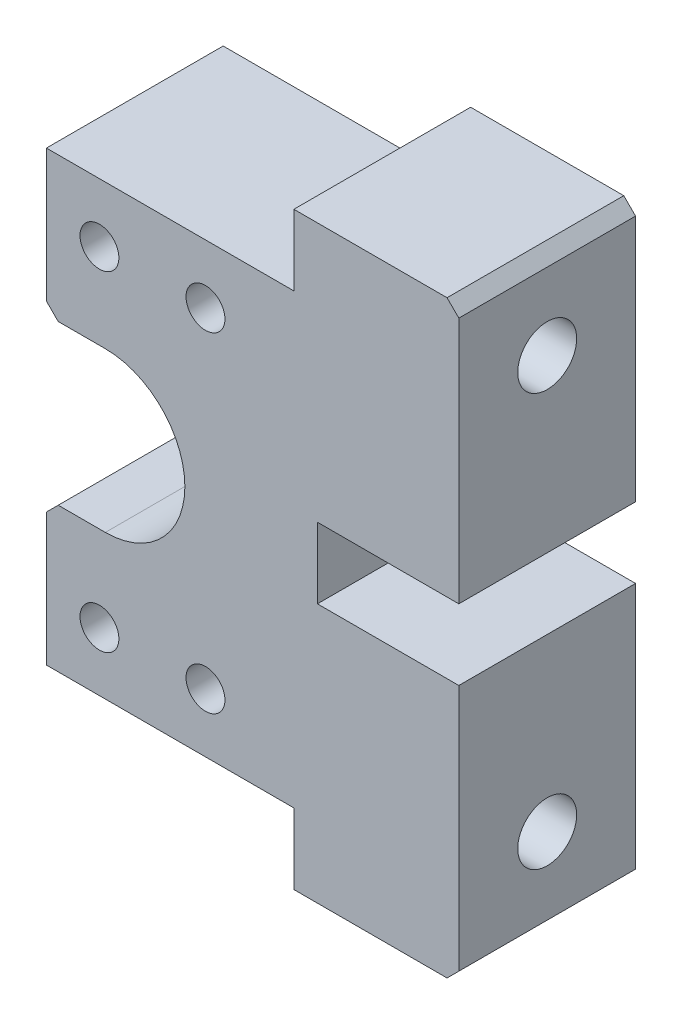
SolidWorks part; units mm, degrees
material "#45(1.1191)"
ref_plane "前视基准面" through (0, 0, 0) normal (0, 0, 1) x (1, 0, 0)
ref_plane "上视基准面" through (0, 0, 0) normal (0, 1, 0) x (1, 0, 0)
ref_plane "右视基准面" through (0, 0, 0) normal (1, 0, 0) x (0, 0, -1)
sketch "草图1" plane through (0, 0, 0) normal (0, 0, 1) x (1, 0, 0)
  line L1 (-17.5, -25) -> (17.5, -25)
  line L2 (-17.5, -25) -> (-17.5, 25)
  line L3 (-17.5, 25) -> (17.5, 25)
  line L4 (17.5, -25) -> (17.5, 25)
  line L5 (-17.5, -25) -> (17.5, 25) construction
  line L6 (-17.5, 25) -> (17.5, -25) construction
  point P0 (0, 0)
  dimension "D1" = 35
  dimension "D2" = 50
extrude "凸台-拉伸1" add sketch "草图1" along normal mid plane 15
sketch "草图2" plane through (0, 0, 7.5) normal (0, 0, 1) x (1, 0, 0)
  line L0 (-17.5, 0) -> (-12.5, 0) construction
  line L1 (-17.5, 25) -> (-17.5, -25) construction
  line L2 (-17.5, 6.75) -> (-12.5, 6.75)
  line L3 (-17.5, -6.75) -> (-12.5, -6.75)
  arc A0 (-17.5, 6.75) -> (-17.5, -6.75) centre (-17.5, 0) ccw
  arc A1 (-12.5, -6.75) -> (-12.5, 6.75) centre (-12.5, 0) ccw
  point P5 (-15, 0)
  dimension "D1" = 13.5
  dimension "D2" = 5
extrude "切除-拉伸1" cut sketch "草图2" against normal through all
sketch "草图7" plane through (0, 0, -7.5) normal (0, 0, -1) x (-1, 0, 0)
  line L0 (-17.5, 0) -> (5.75, 0) construction
  line L1 (-17.5, -25) -> (-17.5, 25) construction
  line L2 (17.5, 25) -> (17.5, 6.75) construction
  line L3 (17.5, -6.75) -> (17.5, -25) construction
  arc A0 (12.5, 6.75) -> (12.5, -6.75) centre (12.5, 0) ccw construction
  point P0 (4, -14)
  point P3 (13, -14)
  point P6 (4, 14)
  point P9 (13, 14)
  dimension "D1" = 14
  dimension "D2" = 14
  dimension "D3" = 14
  dimension "D4" = 14
  dimension "D5" = 4.5
  dimension "D6" = 4.5
  dimension "D7" = 9
  dimension "D8" = 9
hole_wizard "M4 螺纹孔2" positions "草图7" profile "草图8" tap size "M4" standard "ISO" end condition through all
sketch "草图8" plane through (-4, -14, -7.5) normal (1, 0, 0) x (0, 1, 0)
  line L0 (0, 0) -> (0, 15)
  line L1 (0, 15) -> (1.65, 15)
  line L2 (1.65, 15) -> (1.65, 0)
  line L5 (1.65, 0) -> (0, 0)
  line L11 (0, -6.35) -> (0, 107.95) construction
  dimension "通孔螺纹孔钻头直径" = 3.3
  dimension "通孔螺纹孔钻头深度" = 15
cosmetic thread "孔螺蚊线1" parameters "D2"=4
cosmetic thread "孔螺蚊线2" parameters "D2"=4
cosmetic thread "孔螺蚊线3" parameters "D2"=4
cosmetic thread "孔螺蚊线4" parameters "D2"=4
chamfer "倒角1" distance 1 angle 45 4 edges at (17.5, 25, 0) (17.5, -25, 0) (-17.5, -6.75, 0) (-17.5, 6.75, 0)
sketch "草图11" plane through (17.5, 0, 0) normal (1, 0, 0) x (0, 0, -1)
  line L0 (0, -17.5) -> (0, 0) construction
  line L1 (0, 0) -> (0, 17.5) construction
  point P0 (0, -17.5)
  point P5 (0, 17.5)
  dimension "D1" = 35
hole_wizard "M6 螺纹孔1" positions "草图11" profile "草图12" tap size "M6" standard "ISO"
sketch "草图12" plane through (17.5, -17.5, 0) normal (0, 1, 0) x (0, 0, -1)
  line L0 (0, 0) -> (0, 16.5022)
  line L1 (0, 16.5022) -> (2.5, 15)
  line L2 (2.5, 15) -> (2.5, 0)
  line L5 (2.5, 0) -> (0, 0)
  line L10 (0, 16.5022) -> (-2.5, 15) construction
  line L11 (0, -6.35) -> (0, 107.95) construction
  dimension "螺纹孔钻头直径" = 5
  dimension "螺纹孔钻头深度" = 15
  dimension "导头角度" = 118
cosmetic thread "孔螺蚊线5" parameters "D1"=12, "D2"=6
cosmetic thread "孔螺蚊线7" parameters "D1"=12, "D2"=6
sketch "草图15" plane through (17.5, 0, 0) normal (1, 0, 0) x (0, 0, -1)
  point P0 (0, 0)
hole_wizard "Ø6.0mm 暗销孔1" positions "草图15" profile "草图16" hole size "Ø6.0" standard "ISO"
sketch "草图16" plane through (17.5, 0, 0) normal (0, 1, 0) x (0, 0, -1)
  line L0 (0, 0) -> (0, 8.8026)
  line L1 (0, 8.8026) -> (3, 7)
  line L2 (3, 7) -> (3, 0)
  line L5 (3, 0) -> (0, 0)
  line L10 (0, 8.8026) -> (-3, 7) construction
  line L11 (0, -6.35) -> (0, 107.95) construction
  dimension "孔直径" = 6
  dimension "孔深度" = 7
  dimension "导头角度" = 118
sketch "草图17" plane through (0, 0, 7.5) normal (0, 0, 1) x (1, 0, 0)
  line L1 (5.5, 3) -> (17.5, 3)
  line L2 (5.5, 3) -> (5.5, -3)
  line L3 (5.5, -3) -> (17.5, -3)
  line L4 (17.5, 3) -> (17.5, -3)
  line L5 (5.5, 3) -> (17.5, -3) construction
  line L6 (5.5, -3) -> (17.5, 3) construction
  line L7 (0, 0) -> (5.5, 0) construction
  line L8 (17.5, -24) -> (17.5, 24) construction
  point P0 (11.5, 0)
  dimension "D1" = 12
  dimension "D2" = 6
extrude "切除-拉伸2" cut sketch "草图17" against normal through all
chamfer "倒角2" [suppressed] distance 0.5 angle 45
sketch "草图19" plane through (0, 0, 7.5) normal (0, 0, 1) x (1, 0, 0)
  line L1 (-17.5, -25) -> (3.5, -25)
  line L2 (-17.5, -25) -> (-17.5, -19)
  line L3 (-17.5, -19) -> (3.5, -19)
  line L4 (3.5, -25) -> (3.5, -19)
  line L5 (-17.5, 19) -> (3.5, 19)
  line L6 (-17.5, 19) -> (-17.5, 25)
  line L7 (-17.5, 25) -> (3.5, 25)
  line L8 (3.5, 19) -> (3.5, 25)
  dimension "D1" = 21
  dimension "D2" = 38
extrude "切除-拉伸8" cut sketch "草图19" against normal through all
